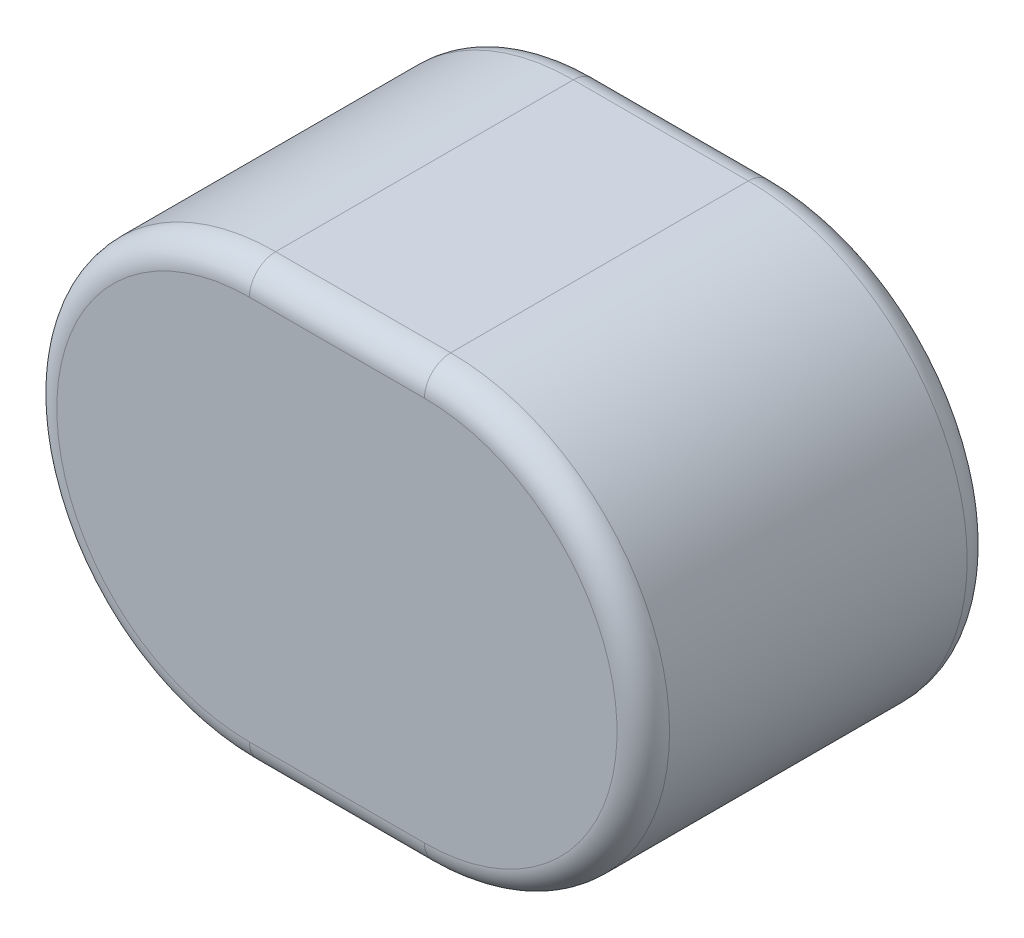
from build123d import *

# Parameters (mm, degrees)
EXTRUDE_523_DEPTH = 8
FILLET_1_R        = 0.6


with BuildPart() as part:
    # 草图1 → Extrude 523 (new body)
    with BuildSketch(Plane.XY):
        with BuildLine():
            Line((-2, 5), (2, 5))
            ThreePointArc((2, 5), (7, 0), (2, -5))
            Line((2, -5), (-2, -5))
            ThreePointArc((-2, -5), (-7, 0), (-2, 5))
        make_face()
    extrude(amount=EXTRUDE_523_DEPTH)

    # 圆角1
    fillet_1_edges = [part.edges().sort_by_distance(p)[0] for p in [
        (7, 0, 8),
        (0, 5, 8),
        (-7, 0, 8),
        (0, 5, 0),
        (7, 0, 0),
        (0, -5, 0),
        (-7, 0, 0),
        (0, -5, 8),
    ]]
    fillet(fillet_1_edges, radius=FILLET_1_R)


solid = part.part
